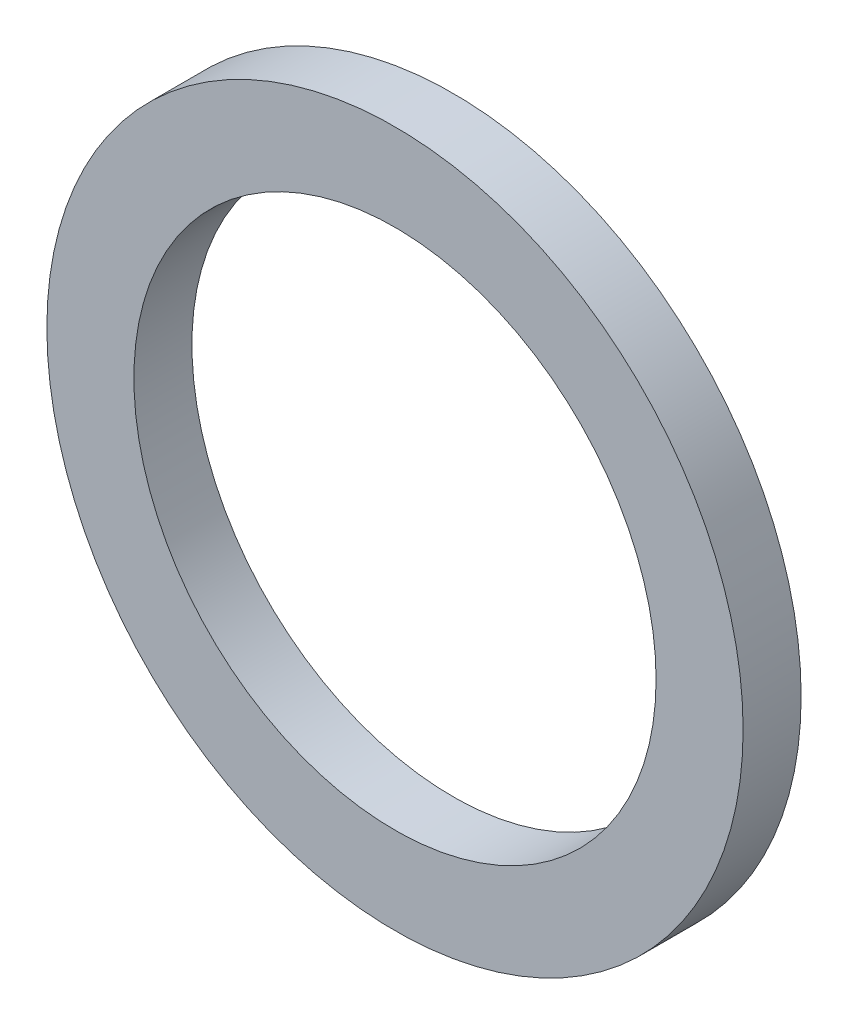
from build123d import *

# Parameters (mm, degrees)
SKETCH1_R           = 30
SKETCH1_R_2         = 22.5
BOSS_EXTRUDE1_DEPTH = 5


with BuildPart() as part:
    # Sketch1 → Boss-Extrude1 (new body)
    with BuildSketch(Plane.XY):
        Circle(SKETCH1_R)
        Circle(SKETCH1_R_2, mode=Mode.SUBTRACT)
    extrude(amount=BOSS_EXTRUDE1_DEPTH)


solid = part.part
